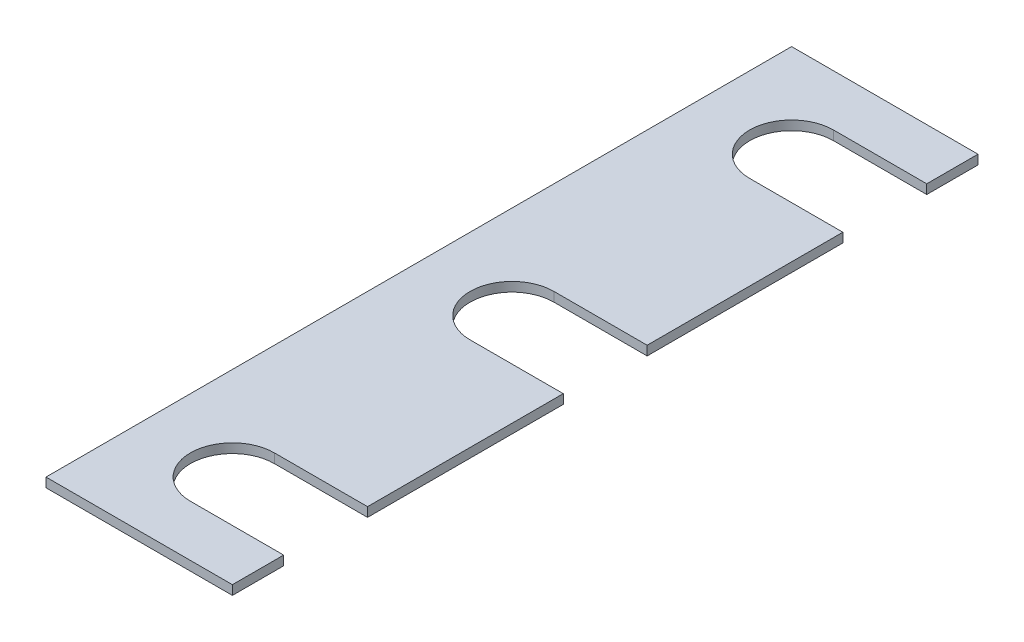
SolidWorks part; units mm, degrees
material "A3"
ref_plane "前视基准面" through (0, 0, 0) normal (0, 0, 1) x (1, 0, 0)
ref_plane "上视基准面" through (0, 0, 0) normal (0, 1, 0) x (1, 0, 0)
ref_plane "右视基准面" through (0, 0, 0) normal (1, 0, 0) x (0, 0, -1)
sketch "草图1" plane through (0, 0, 0) normal (0, 1, 0) x (1, 0, 0)
  line L0 (0, 9) -> (20, 9)
  line L1 (20, 9) -> (20, 51)
  line L2 (20, 51) -> (0, 51)
  line L3 (20, 30) -> (0, 30) construction
  line L4 (0, 69) -> (20, 69)
  line L5 (20, 69) -> (20, 80)
  line L6 (20, 80) -> (-20, 80)
  line L7 (-20, 80) -> (-20, -80)
  line L8 (-20, 0) -> (0, 0) construction
  line L9 (20, -30) -> (0, -30) construction
  line L10 (20, -80) -> (-20, -80)
  line L11 (20, -69) -> (20, -80)
  line L12 (0, -69) -> (20, -69)
  line L13 (20, -51) -> (0, -51)
  line L14 (20, -9) -> (20, -51)
  line L15 (0, -9) -> (20, -9)
  arc A0 (0, 9) -> (0, -9) centre (0, 0) ccw
  arc A1 (0, 51) -> (0, 69) centre (0, 60) cw
  arc A2 (0, -51) -> (0, -69) centre (0, -60) ccw
  dimension "D1" = 18
  dimension "D2" = 20
  dimension "D3" = 42
  dimension "D4" = 40
  dimension "D5" = 20
extrude "凸台-拉伸1" add sketch "草图1" along normal blind 2
